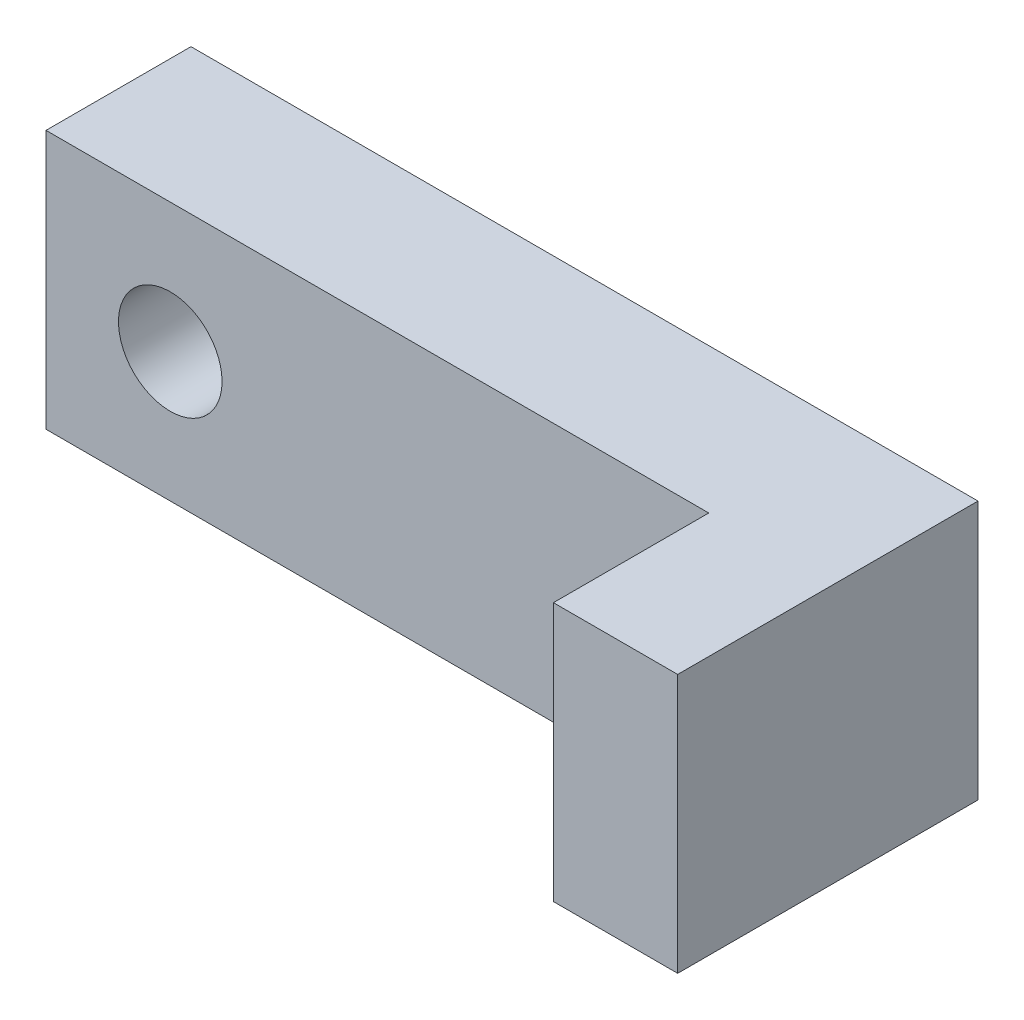
SolidWorks part; units mm, degrees
ref_plane "前视基准面" through (0, 0, 0) normal (0, 0, 1) x (1, 0, 0)
ref_plane "上视基准面" through (0, 0, 0) normal (0, 1, 0) x (1, 0, 0)
ref_plane "右视基准面" through (0, 0, 0) normal (1, 0, 0) x (0, 0, -1)
sketch "草图1" plane through (0, 0, 0) normal (0, 0, 1) x (1, 0, 0)
  line L1 (-38, -12.5) -> (38, -12.5)
  line L2 (-38, -12.5) -> (-38, 12.5)
  line L3 (-38, 12.5) -> (38, 12.5)
  line L4 (38, -12.5) -> (38, 12.5)
  line L5 (-38, -12.5) -> (38, 12.5) construction
  line L6 (-38, 12.5) -> (38, -12.5) construction
  circle A0 centre (-26, 0) radius 5
  point P0 (0, 0)
  dimension "D1" = 10
  dimension "D2" = 64
  dimension "D3" = 12
  dimension "D4" = 25
extrude "凸台-拉伸1" add sketch "草图1" along normal mid plane 14
sketch "草图2" plane through (0, 0, 7) normal (0, 0, 1) x (1, 0, 0)
  line L0 (-38, -12.5) -> (38, -12.5) construction
  line L1 (38, 12.5) -> (26, 12.5)
  line L2 (38, 12.5) -> (38, -12.5)
  line L3 (38, -12.5) -> (26, -12.5)
  line L4 (26, 12.5) -> (26, -12.5)
  dimension "D1" = 12
extrude "凸台-拉伸2" add sketch "草图2" along normal blind 15
